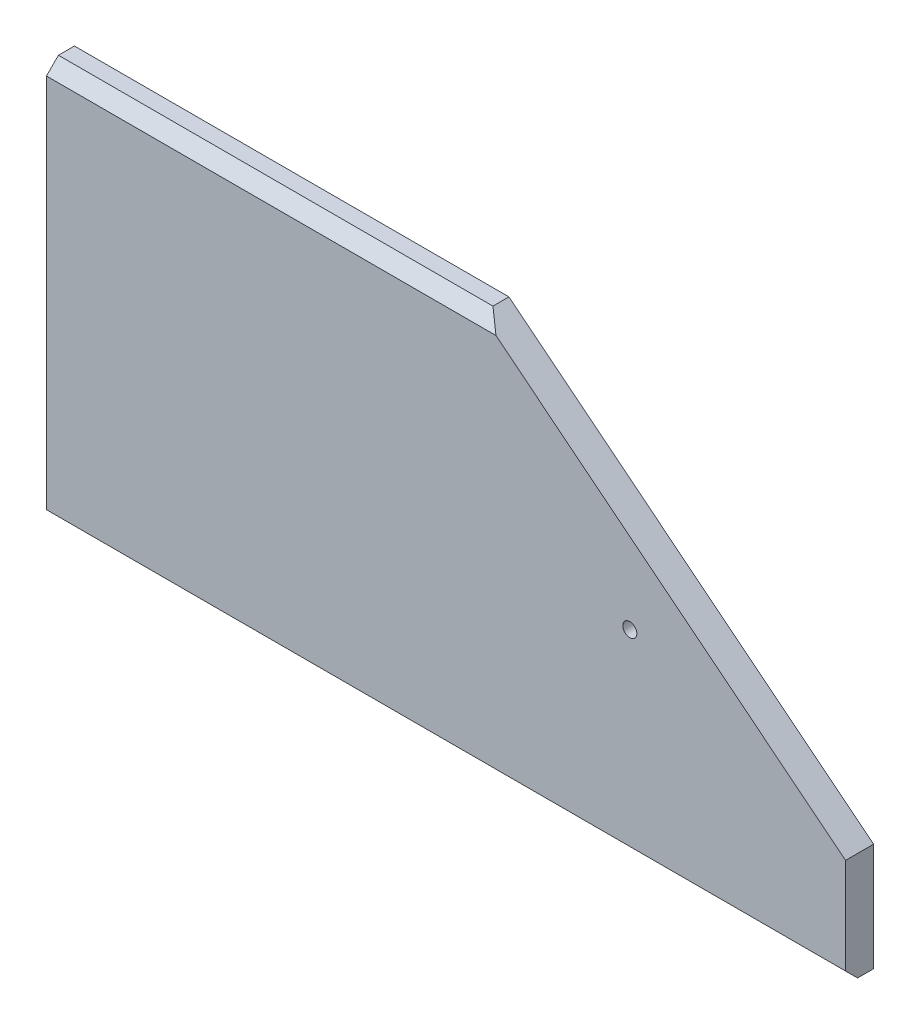
SolidWorks part; units mm, degrees
material "普通碳钢"
ref_plane "Front Plane" through (0, 0, 0) normal (0, 0, 1) x (1, 0, 0)
ref_plane "Top Plane" through (0, 0, 0) normal (0, 1, 0) x (1, 0, 0)
ref_plane "Right Plane" through (0, 0, 0) normal (1, 0, 0) x (0, 0, -1)
sketch "Sketch1" plane through (0, 0, 0) normal (0, 0, 1) x (1, 0, 0)
  line L1 (0, -25) -> (-1000, -25)
  line L2 (0, -25) -> (0, -525)
  line L3 (0, -525) -> (-1000, -525)
  line L4 (-1000, -25) -> (-1000, -525)
  dimension "D1" = 500
  dimension "D2" = 1000
extrude "Boss-Extrude1" add sketch "Sketch1" against normal blind 35
hole_wizard "M20 Tapped Hole1" positions "3DSketch1" profile "Sketch2" tap size "M20" standard "GB" end condition through all
sketch3d "3DSketch1"
  line L0 (0, -275, 0) -> (-1000, -275, 0) construction
  line L1 (0, -525, 0) -> (0, -25, 0) construction
  line L2 (-1000, -25, 0) -> (-1000, -525, 0) construction
  point P0 (-30, -275, 0)
  point P2 (-270, -275, 0)
  dimension "D1" = 30
  dimension "D2" = 240
sketch "Sketch2" plane through (-30, -275, 0) normal (1, 0, 0) x (0, -1, 0)
  line L0 (0, 0) -> (0, 35)
  line L1 (0, 35) -> (8.75, 35)
  line L2 (8.75, 35) -> (8.75, 0)
  line L5 (8.75, 0) -> (0, 0)
  line L11 (0, -6.35) -> (0, 107.95) construction
  dimension "通孔螺纹孔钻头直径" = 17.5
  dimension "通孔螺纹孔钻头深度" = 35
cosmetic thread "Tapped hole thread 1" parameters "D2"=20
cosmetic thread "Tapped hole thread 2" parameters "D2"=20
chamfer "Chamfer1" distance 15 angle 45 2 edges at (-500, -25, 0) (-500, -525, 0)
sketch "Sketch4" plane through (0, 0, 0) normal (0, 0, 1) x (1, 0, 0)
  line L4 (0, -510) -> (0, -40)
  line L5 (0, -40) -> (-1000, -40)
  line L6 (-1000, -40) -> (-1000, -510)
  line L7 (-1000, -510) -> (0, -510)
  line L10 (-1000, -40) -> (-1000, -510)
  line L11 (-1000, -510) -> (0, -510)
  dimension "D1" = 0
sketch "Sketch8" plane through (0, -525, 0) normal (0, -1, 0) x (1, 0, 0)
  line L0 (-500, 0) -> (0, 0)
  line L1 (-1000, 0) -> (0, 0) construction
  line L2 (0, 0) -> (0, -300)
  line L3 (0, -300) -> (-500, 0)
  dimension "D1" = 500
  dimension "D2" = 300
sketch "Sketch9" plane through (0, 0, 0) normal (0, 0, 1) x (1, 0, 0)
  line L0 (-500, 10) -> (0, 10)
  line L2 (0, 10) -> (0, -390)
  line L3 (0, -510) -> (0, -40) construction
  line L4 (0, -390) -> (-500, 10)
  line L5 (-1000, -25) -> (0, -25) construction
  dimension "D1" = 500
  dimension "D2" = 400
  dimension "D3" = 35
extrude "Cut-Extrude3" cut sketch "Sketch9" against normal through all
